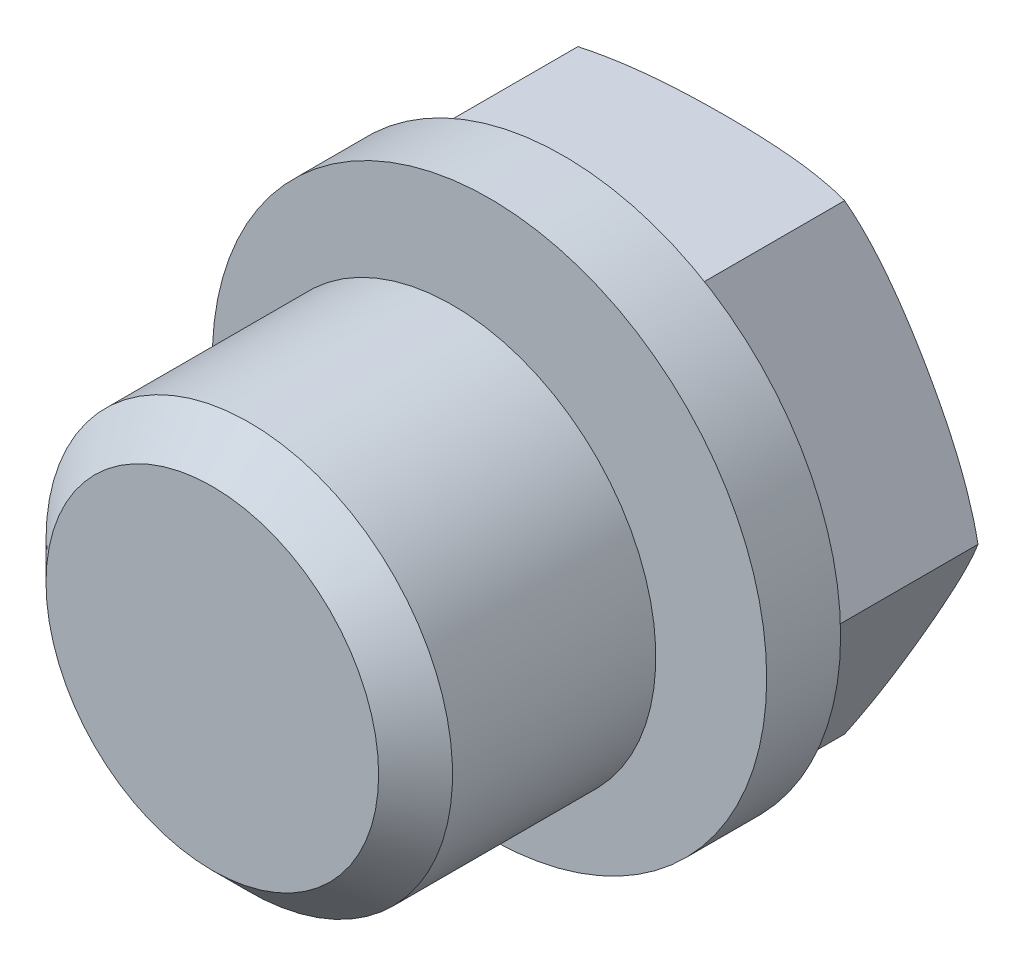
from build123d import *

# Parameters (mm, degrees)
BOSS_EXTRUDE1_DEPTH = 9
SKETCH2_R           = 15
BOSS_EXTRUDE2_DEPTH = 4
SKETCH3_R           = 7.5
BOSS_EXTRUDE3_DEPTH = 2
SKETCH4_R           = 11
BOSS_EXTRUDE5_DEPTH = 13
CHAMFER1_SIZE       = 2
SCALE_1_SCALE       = 1.875


with BuildPart() as part:
    # Sketch1 → Boss-Extrude1 (new body)
    with BuildSketch(Plane.XY):
        Polygon((14.43375673, 0), (7.216878365, 12.5), (-7.216878365, 12.5), (-14.43375673, 0), (-7.216878365, -12.5), (7.216878365, -12.5), align=None)
    extrude(amount=BOSS_EXTRUDE1_DEPTH)

    # Sketch2 → Boss-Extrude2 (add)
    with BuildSketch(Plane.XY.offset(9)):
        Circle(SKETCH2_R)
    extrude(amount=BOSS_EXTRUDE2_DEPTH)

    # Sketch3 → Boss-Extrude3 (add)
    with BuildSketch(Plane.XY.offset(13)):
        Circle(SKETCH3_R)
    extrude(amount=BOSS_EXTRUDE3_DEPTH)

    # Sketch4 → Boss-Extrude5 (add)
    with BuildSketch(Plane.XY.offset(15)):
        with Locations(Location((0, 0, 0), (0, 0, 180))):
            Circle(SKETCH4_R)
    extrude(amount=BOSS_EXTRUDE5_DEPTH)

    # Chamfer1
    chamfer1_edges = [part.edges().sort_by_distance(p)[0] for p in [
        (11, 0, 28),
    ]]
    chamfer(chamfer1_edges, length=CHAMFER1_SIZE)

    # Sketch6 → Cut-Revolve4 (revolve, cut)
    with BuildSketch(Plane(origin=(0, 0, 0), x_dir=(1, 0, 0), z_dir=(0, 1, 0)), mode=Mode.PRIVATE) as cut_revolve4_sk:
        with BuildLine():
            Line((-10.43375673, 0), (-11.300713231, 3.45481125))
            Line((-11.300713231, 3.45481125), (-14.43375673, 0))
            Line((-14.43375673, 0), (-14.43375673, -1))
            ThreePointArc((-14.43375673, -1), (-12.499286844, -0.237879543), (-10.43375673, 0))
        make_face()
    revolve(cut_revolve4_sk.sketch.rotate(Axis((0, 0, 0), (0, 0, -1)), 180), axis=Axis((0, 0, 0), (0, 0, -1)), mode=Mode.SUBTRACT)


with BuildPart() as part_1:
    # Scale 1: scaled about (-3.1e-08, 2.41e-07, 12.521211358)
    add(part.part.scale(SCALE_1_SCALE).moved(Location((2.7e-08, -2.11e-07, -10.956059938))))


solid = part_1.part
